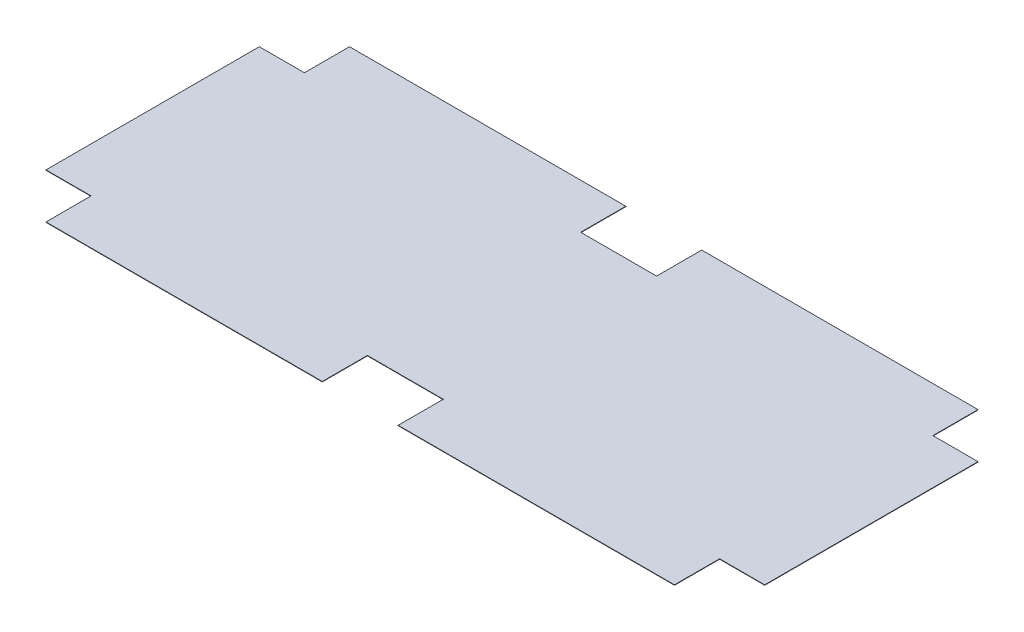
SolidWorks part; units mm, degrees
ref_plane "Front Plane" through (0, 0, 0) normal (0, 0, 1) x (1, 0, 0)
ref_plane "Top Plane" through (0, 0, 0) normal (0, 1, 0) x (1, 0, 0)
ref_plane "Right Plane" through (0, 0, 0) normal (1, 0, 0) x (0, 0, -1)
sketch "Sketch 1" plane through (0, 0, 0) normal (0, 1, 0) x (1, 0, 0)
  line L0 (0, 1610.1852) -> (0, -1740.3704) construction
  line L1 (-3495.168, 0) -> (3807.744, 0) construction
  line L2 (2195, 1060) -> (265, 1060)
  line L3 (-2195, 1060) -> (-2195, 745)
  line L4 (-2195, 745) -> (-2510, 745)
  line L5 (-2510, 745) -> (-2510, -745)
  line L6 (-2195, -745) -> (-2510, -745)
  line L7 (-2195, -1060) -> (-2195, -745)
  line L8 (2195, -1060) -> (265, -1060)
  line L9 (2195, -1060) -> (2195, -745)
  line L10 (2195, -745) -> (2510, -745)
  line L11 (2510, 745) -> (2510, -745)
  line L12 (2195, 745) -> (2510, 745)
  line L13 (2195, 1060) -> (2195, 745)
  line L14 (-265, 1060) -> (-265, 745)
  line L15 (-265, 745) -> (265, 745)
  line L16 (265, 1060) -> (265, 745)
  line L17 (265, -1060) -> (265, -745)
  line L18 (-265, -745) -> (265, -745)
  line L19 (-265, -1060) -> (-265, -745)
  line L20 (-265, 1060) -> (-2195, 1060)
  line L21 (-265, -1060) -> (-2195, -1060)
  point P5 (2510, 0)
  point P13 (-2510, 0)
  point P17 (0, -1060)
  point P22 (0, 1060)
  point P25 (0, 745)
  dimension "D1" = 315
  dimension "D2" = 4390
  dimension "D3" = 5020
  dimension "D4" = 2120
  dimension "D5" = 265
extrude "Boss-Extrude 1" add sketch "Sketch 1" along normal blind 3
